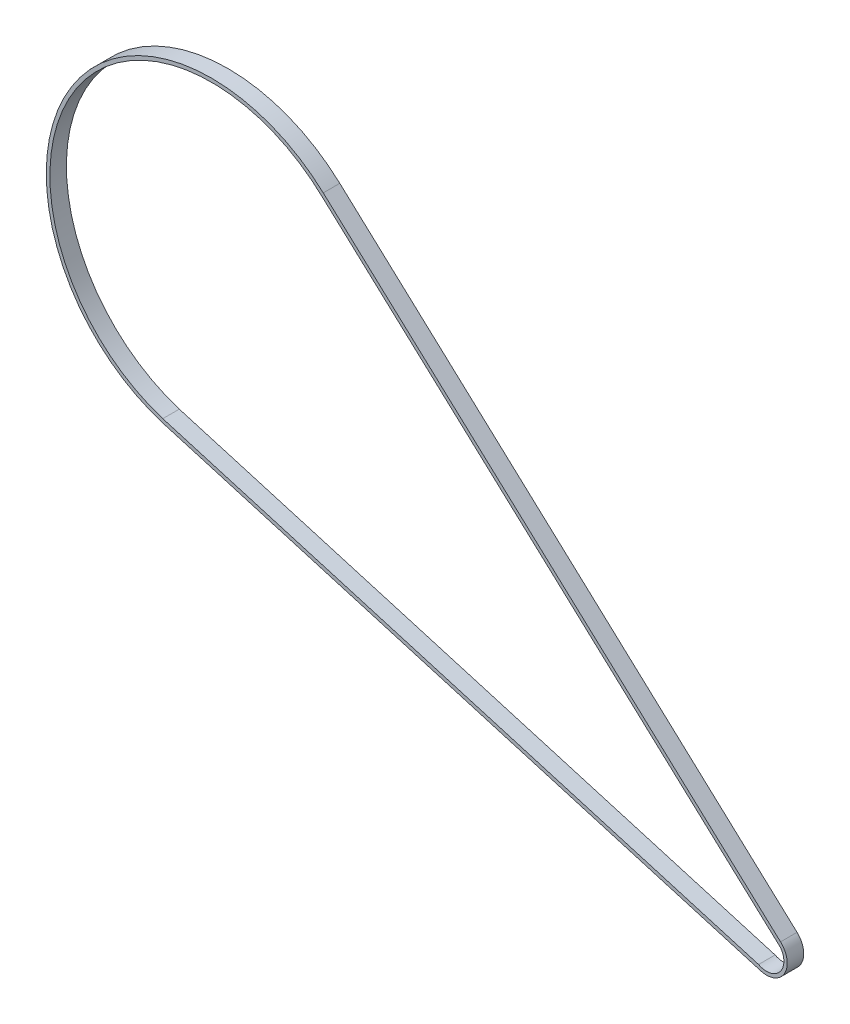
from build123d import *

# Parameters (mm, degrees)
SKETCH2_W = 20
SKETCH2_H = 6


with BuildPart() as part:
    # Sweep1: sweep along a path in Sketch1
    with BuildLine(Plane.XY) as sweep1_path:
        Line((-460.524027919, 638.205508164), (92.975879138, 129.813393739))
        ThreePointArc((92.975879138, 129.813393739), (97.831928599, 99.10611839), (69.02602264, 87.412626283))
        Line((69.02602264, 87.412626283), (-652.122879897, 298.999368519))
        ThreePointArc((-652.122879897, 298.999368519), (-769.956329171, 589.271874597), (-460.524027919, 638.205508164))
    # Sketch2 → Sweep1 (sweep)
    with BuildSketch(Plane(origin=(-460.524027919, 0, 0), x_dir=(0, 0, -1), z_dir=(1, 0, 0))):
        with Locations((0, 635.205508164)):
            Rectangle(SKETCH2_W, SKETCH2_H)
    sweep(path=sweep1_path.line)


solid = part.part
